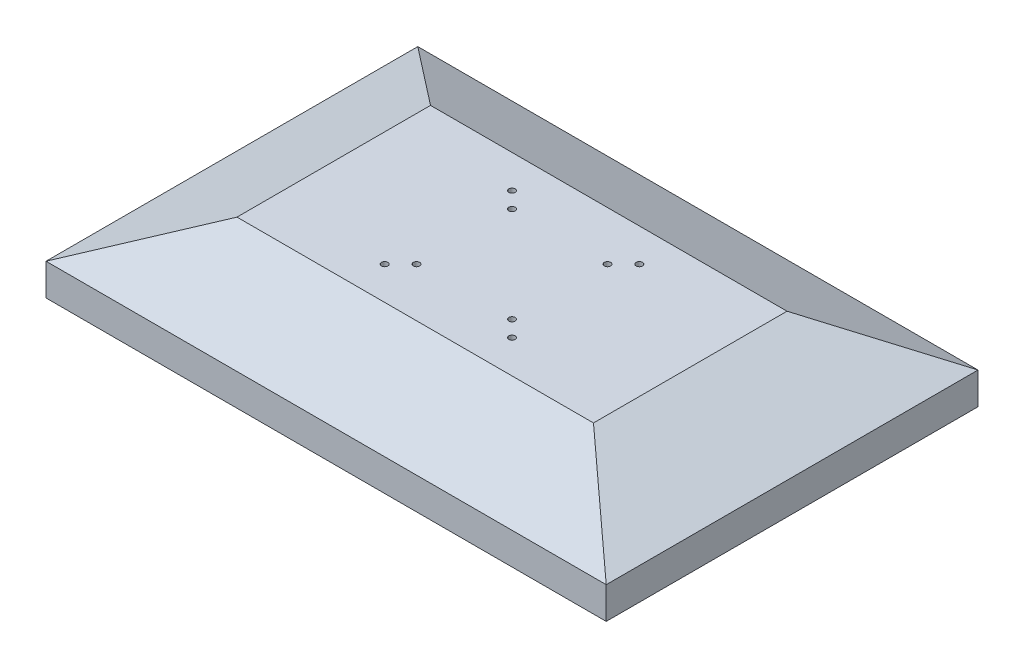
from build123d import *

# Parameters (mm, degrees)
SKETCH_1_W          = 440
SKETCH_1_H          = 292
EXTRUDE_1_DEPTH     = 60
CUT_EXTRUDE_1_DEPTH = 379
CUT_EXTRUDE_2_DEPTH = 467
SKETCH_5_R          = 2.5
CUT_EXTRUDE_3_DEPTH = 20


with BuildPart() as part:
    # 草图1 → 凸台-拉伸1 (new body)
    with BuildSketch(Plane(origin=(0, 0, 0), x_dir=(1, 0, 0), z_dir=(0, 1, 0))):
        with Locations((220, 146)):
            Rectangle(SKETCH_1_W, SKETCH_1_H)
    extrude(amount=EXTRUDE_1_DEPTH)

    # 草图3 → 切除-拉伸1 (cut)
    with BuildSketch(Plane(origin=(0, 0, -292), x_dir=(-1, 0, 0), z_dir=(0, 0, -1))):
        Polygon((-440, 60), (-440, 25), (-360, 60), align=None)
        Polygon((-80, 60), (0, 25), (0, 60), align=None)
    extrude(amount=-CUT_EXTRUDE_1_DEPTH, mode=Mode.SUBTRACT)

    # 草图4 → 切除-拉伸2 (cut)
    with BuildSketch(Plane.ZY):
        Polygon((-292, 60), (-292, 25), (-222, 60), align=None)
        Polygon((-70, 60), (0, 25), (0, 60), align=None)
    extrude(amount=-CUT_EXTRUDE_2_DEPTH, mode=Mode.SUBTRACT)

    # 草图5 → 切除-拉伸3 (cut)
    with BuildSketch(Plane(origin=(0, 60, 0), x_dir=(1, 0, 0), z_dir=(0, 1, 0))):
        with Locations(Location((270, 196, 0), (0, 0, 270))):
            Circle(SKETCH_5_R)
        with Locations(Location((257.5, 183.5, 0), (0, 0, 270))):
            Circle(SKETCH_5_R)
        with Locations(Location((270, 96, 0), (0, 0, 270))):
            Circle(SKETCH_5_R)
        with Locations(Location((257.5, 108.5, 0), (0, 0, 270))):
            Circle(SKETCH_5_R)
        with Locations(Location((170, 96, 0), (0, 0, 270))):
            Circle(SKETCH_5_R)
        with Locations(Location((182.5, 108.5, 0), (0, 0, 270))):
            Circle(SKETCH_5_R)
        with Locations(Location((170, 196, 0), (0, 0, 270))):
            Circle(SKETCH_5_R)
        with Locations(Location((182.5, 183.5, 0), (0, 0, 270))):
            Circle(SKETCH_5_R)
    extrude(amount=-CUT_EXTRUDE_3_DEPTH, mode=Mode.SUBTRACT)


solid = part.part
